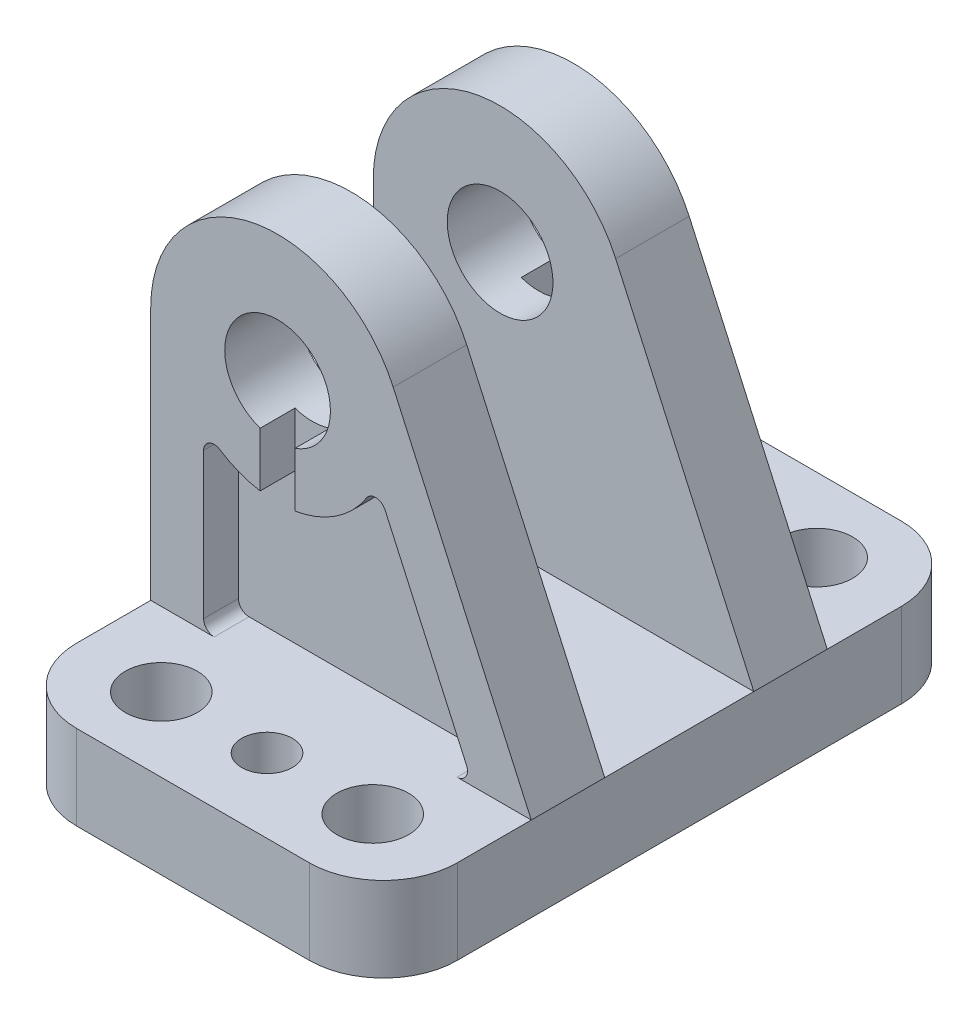
SolidWorks part; units mm, degrees
ref_plane "前视基准面" through (0, 0, 0) normal (0, 0, 1) x (1, 0, 0)
ref_plane "上视基准面" through (0, 0, 0) normal (0, 1, 0) x (1, 0, 0)
ref_plane "右视基准面" through (0, 0, 0) normal (1, 0, 0) x (0, 0, -1)
ref_plane "基准面4" through (0, 0, -14) normal (0, 0, -1) x (-1, 0, 0)
sketch "草图1" plane through (0, 0, -14) normal (0, 0, -1) x (-1, 0, 0)
  line L0 (-4.9373, 36.9373) -> (-18, 8)
  line L1 (-18, 8) -> (18, 8)
  line L2 (18, 8) -> (18, 32)
  arc A0 (18, 32) -> (-4.9373, 36.9373) centre (6, 32) ccw
extrude "凸台-拉伸1" add sketch "草图1" against normal blind 6.95
sketch "草图2" plane through (0, 8, 0) normal (0, -1, 0) x (1, 0, 0)
  line L0 (-18, -7.05) -> (18, -7.05)
  line L1 (18, -7.05) -> (18, -14)
  line L2 (18, -14) -> (-18, -14)
  line L3 (-18, -14) -> (-18, -7.05)
extrude "凸台-拉伸2" add sketch "草图2" along normal blind 8
sketch "草图3" plane through (0, 0, -7.05) normal (0, 0, 1) x (1, 0, 0)
  line L0 (-18, 0) -> (-18, 8)
  line L1 (-18, 8) -> (18, 8)
  line L2 (18, 8) -> (18, 0)
  line L3 (18, 0) -> (-18, 0)
extrude "凸台-拉伸3" add sketch "草图3" along normal blind 14.1
sketch "草图4" plane through (0, 0, 7.05) normal (0, 0, 1) x (1, 0, 0)
  line L0 (-18, 0) -> (-18, 32)
  line L1 (4.9373, 36.9373) -> (18, 8)
  line L2 (18, 8) -> (18, 0)
  line L3 (18, 0) -> (-18, 0)
  arc A0 (-18, 32) -> (4.9373, 36.9373) centre (-6, 32) cw
extrude "凸台-拉伸4" add sketch "草图4" along normal blind 6.95
sketch "草图5" plane through (0, 0, 14) normal (0, 0, 1) x (1, 0, 0)
  line L0 (-18, 8) -> (18, 8)
  line L1 (18, 8) -> (18, 0)
  line L2 (18, 0) -> (-18, 0)
  line L3 (-18, 0) -> (-18, 8)
extrude "凸台-拉伸5" add sketch "草图5" along normal blind 14
sketch "草图6" plane through (0, 0, 14) normal (0, 0, 1) x (1, 0, 0)
  line L0 (-13, 22.7805) -> (-13, 8)
  line L1 (-13, 8) -> (10.9656, 8)
  line L2 (11.877, 9.4114) -> (4.1733, 26.477)
  arc A0 (2.4199, 26.6051) -> (-11.4545, 23.6186) centre (-6, 32) cw
  arc A1 (-11.4545, 23.6186) -> (-13, 22.7805) centre (-12, 22.7805) ccw
  arc A2 (10.9656, 8) -> (11.877, 9.4114) centre (10.9656, 9) ccw
  arc A3 (4.1733, 26.477) -> (2.4199, 26.6051) centre (3.2619, 26.0656) ccw
extrude "切除-拉伸1" cut sketch "草图6" against normal blind 3.3
sketch "草图7" plane through (0, 0, -14) normal (0, 0, -1) x (-1, 0, 0)
  line L0 (-18, 8) -> (18, 8)
  line L1 (18, 8) -> (18, 0)
  line L2 (18, 0) -> (-18, 0)
  line L3 (-18, 0) -> (-18, 8)
extrude "凸台-拉伸6" add sketch "草图7" along normal blind 14
sketch "草图8" plane through (0, 0, -14) normal (0, 0, -1) x (-1, 0, 0)
  line L0 (-4.1733, 26.477) -> (-11.877, 9.4114)
  line L1 (-10.9656, 8) -> (13, 8)
  line L2 (13, 8) -> (13, 22.7805)
  arc A0 (13, 22.7805) -> (11.4545, 23.6186) centre (12, 22.7805) ccw
  arc A1 (11.4545, 23.6186) -> (-2.4199, 26.6051) centre (6, 32) cw
  arc A2 (-2.4199, 26.6051) -> (-4.1733, 26.477) centre (-3.2619, 26.0656) ccw
  arc A3 (-11.877, 9.4114) -> (-10.9656, 8) centre (-10.9656, 9) ccw
extrude "切除-拉伸2" cut sketch "草图8" against normal blind 3.3
sketch "草图9" plane through (0, 0, 14) normal (0, 0, 1) x (1, 0, 0)
  line L0 (-7.65, 27.2801) -> (-7.65, 22.1371)
  line L1 (-4.35, 22.1371) -> (-4.35, 27.2801)
  arc A0 (-7.65, 22.1371) -> (-4.35, 22.1371) centre (-6, 32) ccw
  arc A1 (-4.35, 27.2801) -> (-7.65, 27.2801) centre (-6, 32) cw
extrude "切除-拉伸3" cut sketch "草图9" against normal blind 3.3
sketch "草图10" plane through (0, 0, -14) normal (0, 0, -1) x (-1, 0, 0)
  line L0 (7.65, 22.1371) -> (7.65, 27.2801)
  line L1 (4.35, 27.2801) -> (4.35, 22.1371)
  arc A0 (4.35, 22.1371) -> (7.65, 22.1371) centre (6, 32) ccw
  arc A1 (7.65, 27.2801) -> (4.35, 27.2801) centre (6, 32) cw
extrude "切除-拉伸4" cut sketch "草图10" against normal blind 3.3
sketch "草图11" plane through (0, 0, 0) normal (0, -1, 0) x (1, 0, 0)
  line L0 (-13, 14.2354) -> (-13, -14.2354)
  line L1 (-4.1255, -16.5) -> (4.1255, -16.5)
  line L2 (13, -14.2354) -> (13, 14.2354)
  line L3 (4.1255, 16.5) -> (-4.1255, 16.5)
  arc A0 (-4.1255, 16.5) -> (-13, 14.2354) centre (-10, 21) cw
  arc A1 (-13, -14.2354) -> (-4.1255, -16.5) centre (-10, -21) cw
  arc A2 (4.1255, -16.5) -> (13, -14.2354) centre (10, -21) cw
  arc A3 (13, 14.2354) -> (4.1255, 16.5) centre (10, 21) cw
extrude "切除-拉伸5" cut sketch "草图11" against normal blind 4
ref_plane "基准面5" through (0, 32, 0) normal (0, 1, 0) x (1, 0, 0)
sketch "草图12" plane through (0, 32, 0) normal (0, 1, 0) x (1, 0, 0)
  line L0 (-1, -7.05) -> (-6, -7.05)
  line L1 (-6, -7.05) -> (-6, -14)
  line L2 (-6, -14) -> (-1, -14)
  line L3 (-1, -14) -> (-1, -7.05)
  line L4 (-6, -7.05) -> (-6, -14) construction
revolve "切除-旋转1" cut sketch "草图12" angle 360 about L4
ref_plane "基准面6" through (0, 32, 0) normal (0, -1, 0) x (1, 0, 0)
sketch "草图13" plane through (0, 32, 0) normal (0, -1, 0) x (1, 0, 0)
  line L0 (-1, -7.05) -> (-6, -7.05)
  line L1 (-6, -7.05) -> (-6, -14)
  line L2 (-6, -14) -> (-1, -14)
  line L3 (-1, -14) -> (-1, -7.05)
  line L4 (-6, -7.05) -> (-6, -14) construction
revolve "切除-旋转2" cut sketch "草图13" angle 360 about L4
hole_wizard "Ø4.8 (4.8) 直径孔1" positions "草图15" profile "草图14" hole size "Ø4.8" standard "ANSI Metric"
sketch "草图15" plane through (0, 0, 0) normal (0, -1, 0) x (-1, 0, 0)
  point P0 (0, 21)
  point P1 (0, -21)
sketch "草图14" plane through (0, 0, -21) normal (1, 0, 0) x (0, 0, -1)
  line L0 (0, 0) -> (0, 44)
  line L1 (0, 44) -> (2.4, 44)
  line L2 (2.4, 44) -> (2.4, 0)
  line L5 (2.4, 0) -> (0, 0)
  line L11 (0, -6.35) -> (0, 107.95) construction
  dimension "通孔孔直径" = 4.8
  dimension "通孔孔深度" = 44
hole_wizard "Ø6.8 (6.8) 直径孔1" positions "草图17" profile "草图16" hole size "Ø6.8" standard "ANSI Metric"
sketch "草图17" plane through (0, 0, 0) normal (0, -1, 0) x (-1, 0, 0)
  point P0 (-10, 21)
  point P1 (-10, -21)
  point P2 (10, 21)
  point P3 (10, -21)
sketch "草图16" plane through (10, 0, -21) normal (1, 0, 0) x (0, 0, -1)
  line L0 (0, 0) -> (0, 44)
  line L1 (0, 44) -> (3.4, 44)
  line L2 (3.4, 44) -> (3.4, 0)
  line L5 (3.4, 0) -> (0, 0)
  line L11 (0, -6.35) -> (0, 107.95) construction
  dimension "通孔孔直径" = 6.8
  dimension "通孔孔深度" = 44
fillet "圆角1" radius 1 10 edges at (13, 2, -14.2354) (4.1255, 2, -16.5) (-13, 2, 14.2354) (-4.1255, 2, 16.5) (-13, 2, -14.2354) (-13, 8, -12.35) (13, 2, 14.2354) (-13, 8, 12.35) (4.1255, 2, 16.5) (-4.1255, 2, -16.5)
fillet "圆角2" radius 7 4 edges at (-18, 4, -28) (18, 4, -28) (18, 4, 28) (-18, 4, 28)
